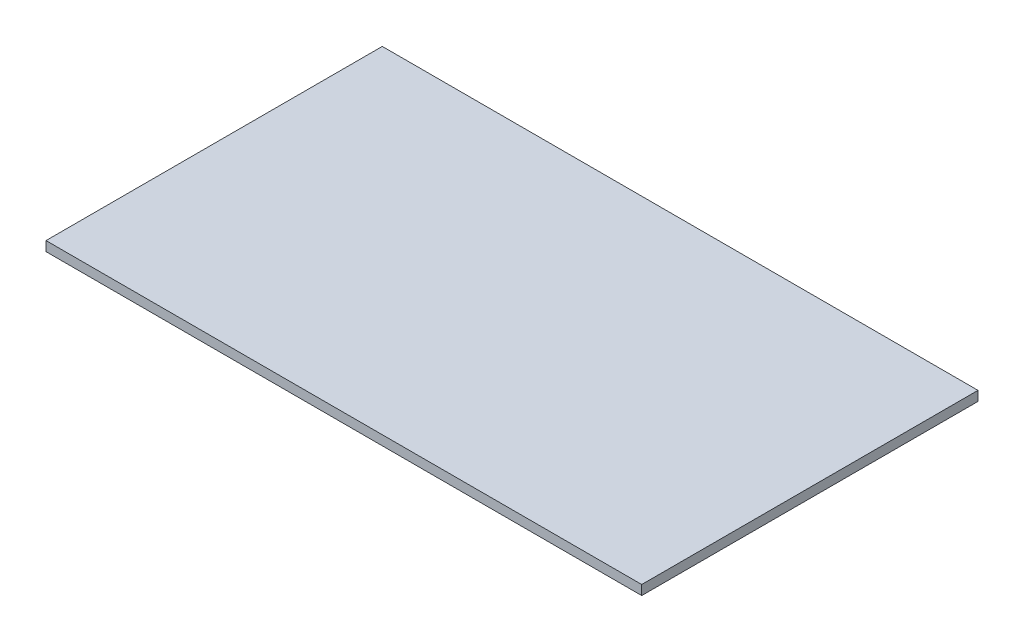
from build123d import *

# Parameters (mm, degrees)
SKETCH1_W           = 6800
SKETCH1_H           = 4800
BOSS_EXTRUDE1_DEPTH = 100
SKETCH2_OUTSIDE_W   = 8466.812
SKETCH2_OUTSIDE_H   = 6466.812
SKETCH2_OUTSIDE_W_2 = 6200
SKETCH2_OUTSIDE_H_2 = 3500
CUT_EXTRUDE1_DEPTH  = 4163.9316593


with BuildPart() as part:
    # Sketch1 → Boss-Extrude1 (new body)
    with BuildSketch(Plane(origin=(0, 0, 0), x_dir=(1, 0, 0), z_dir=(0, 1, 0))):
        Rectangle(SKETCH1_W, SKETCH1_H)
    extrude(amount=BOSS_EXTRUDE1_DEPTH)

    # Sketch2 outside → Cut-Extrude1 (cut, through all)
    with BuildSketch(Plane(origin=(0, 100, 0), x_dir=(1, 0, 0), z_dir=(0, 1, 0))):
        Rectangle(SKETCH2_OUTSIDE_W, SKETCH2_OUTSIDE_H)
        with Locations((-300, 650)):
            Rectangle(SKETCH2_OUTSIDE_W_2, SKETCH2_OUTSIDE_H_2, mode=Mode.SUBTRACT)
    extrude(amount=-CUT_EXTRUDE1_DEPTH, mode=Mode.SUBTRACT)


solid = part.part
